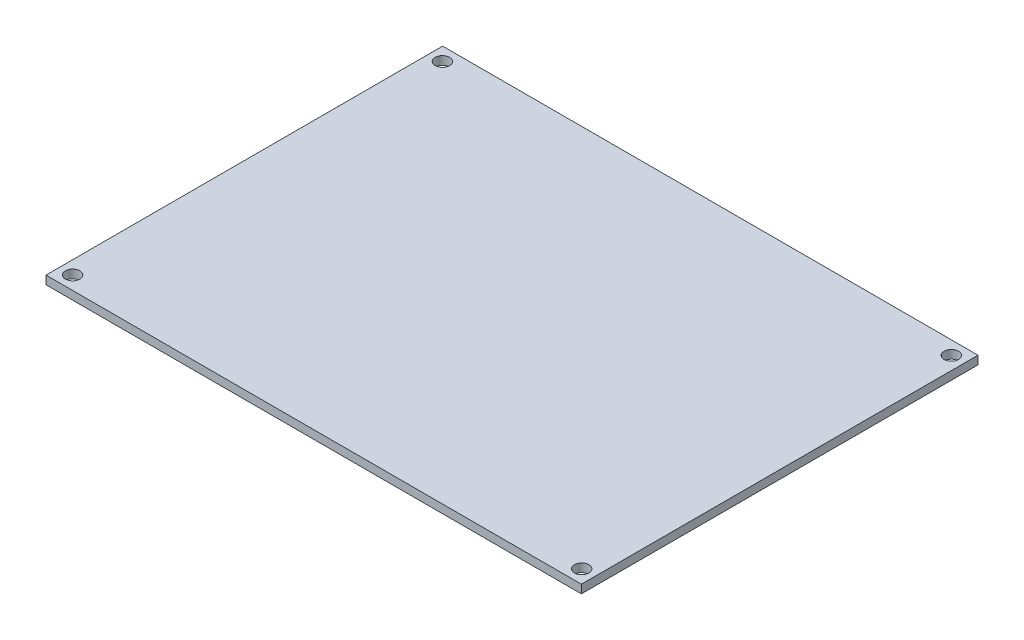
from build123d import *

# Parameters (mm, degrees)
SKETCH_1_W      = 111.5
SKETCH_1_H      = 82.6
SKETCH_1_R      = 1.5
EXTRUDE_1_DEPTH = 1.75


with BuildPart() as part:
    # 草图1 → 凸台-拉伸1 (new body)
    with BuildSketch(Plane(origin=(0, 0, 0), x_dir=(1, 0, 0), z_dir=(0, 1, 0))):
        Rectangle(SKETCH_1_W, SKETCH_1_H)
        with Locations(Location((-53, 38.5, 0), (0, 0, 270))):
            Circle(SKETCH_1_R, mode=Mode.SUBTRACT)
        with Locations(Location((53, 38.5, 0), (0, 0, 90))):
            Circle(SKETCH_1_R, mode=Mode.SUBTRACT)
        with Locations(Location((53, -38.5, 0), (0, 0, 270))):
            Circle(SKETCH_1_R, mode=Mode.SUBTRACT)
        with Locations(Location((-53, -38.5, 0), (0, 0, 90))):
            Circle(SKETCH_1_R, mode=Mode.SUBTRACT)
    extrude(amount=EXTRUDE_1_DEPTH)


solid = part.part
